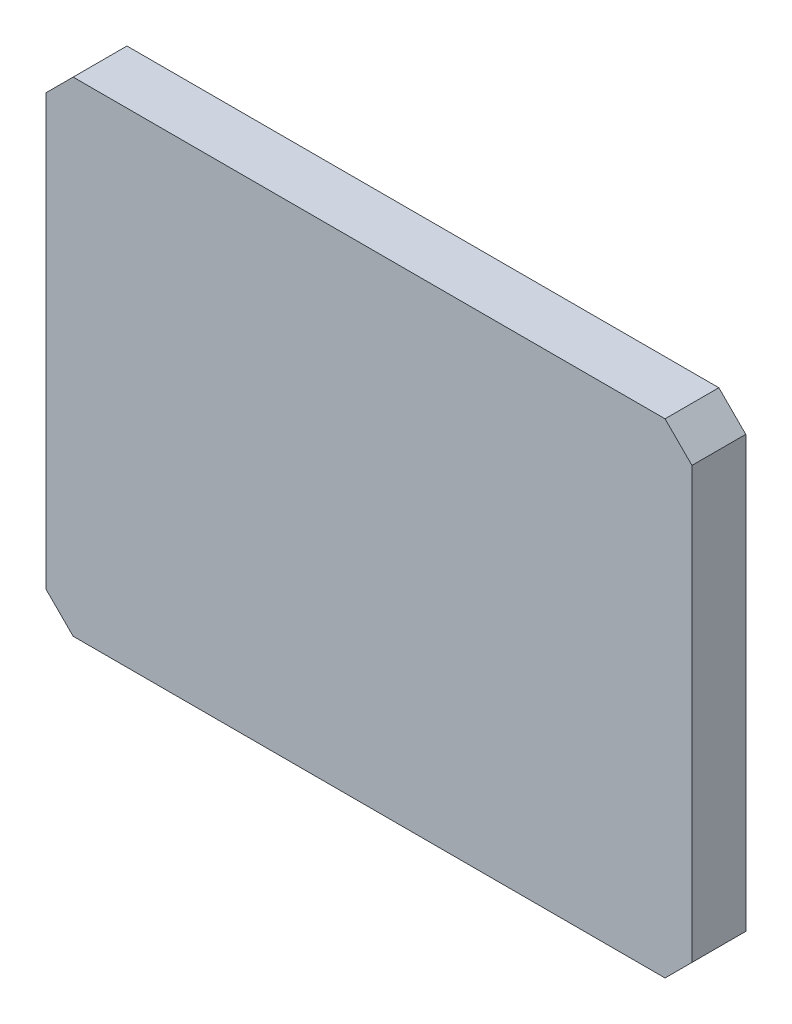
from build123d import *

# Parameters (mm, degrees)
SKETCH1_W           = 120
SKETCH1_H           = 90
BOSS_EXTRUDE1_DEPTH = 10
CHAMFER1_SIZE       = 5


with BuildPart() as part:
    # Sketch1 → Boss-Extrude1 (new body)
    with BuildSketch(Plane.XY):
        Rectangle(SKETCH1_W, SKETCH1_H)
    extrude(amount=BOSS_EXTRUDE1_DEPTH)

    # Chamfer1
    chamfer1_edges = [part.edges().sort_by_distance(p)[0] for p in [
        (-60, 45, 5),
        (60, 45, 5),
        (60, -45, 5),
        (-60, -45, 5),
    ]]
    chamfer(chamfer1_edges, length=CHAMFER1_SIZE)


solid = part.part
